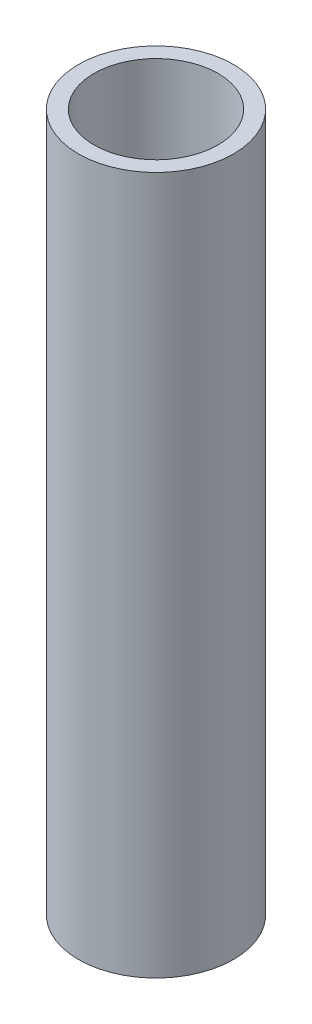
SolidWorks part; units mm, degrees
material "Q235B"
ref_plane "Front Plane" through (0, 0, 0) normal (0, 0, 1) x (1, 0, 0)
ref_plane "Top Plane" through (0, 0, 0) normal (0, 1, 0) x (1, 0, 0)
ref_plane "Right Plane" through (0, 0, 0) normal (1, 0, 0) x (0, 0, -1)
sketch "Sketch1" plane through (0, 0, 0) normal (0, 0, 1) x (1, 0, 0)
  line L0 (0, 0) -> (0, 90)
  dimension "D1" = 90
other "GB/T 6728-2002 round tube 20 × 2(1)"
ref_plane "Plane1" through (0, 0, 0) normal (0, 1, 0) x (-1, 0, 0)
sketch "Sketch11" plane through (0, 0, 0) normal (0, 1, 0) x (-1, 0, 0)
  circle A0 centre (0, 0) radius 8
  circle A1 centre (0, 0) radius 10
  point P3 (0, 0)
  dimension "Out_dia" = 20
  dimension "D1" = 2
